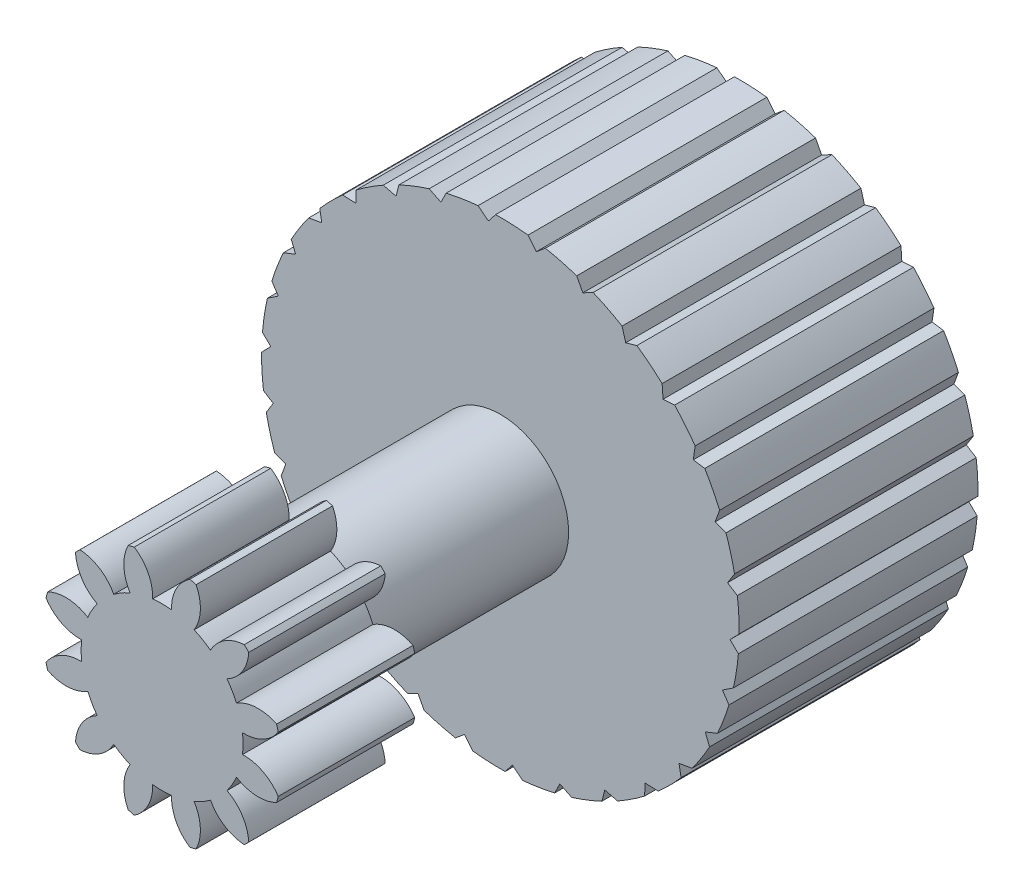
from build123d import *

# Parameters (mm, degrees)
SKETCH1_R           = 1
BOSS_EXTRUDE1_DEPTH = 3
BOSS_EXTRUDE2_DEPTH = 2
SKETCH3_R           = 3.5
BOSS_EXTRUDE3_DEPTH = 3.5
CUT_EXTRUDE1_DEPTH  = 5
CIRPATTERN1_COUNT   = 30
SCALE_1_SCALE       = 0.7


with BuildPart() as part:
    # Sketch1 → Boss-Extrude1 (new body)
    with BuildSketch(Plane.XY):
        Circle(SKETCH1_R)
    extrude(amount=BOSS_EXTRUDE1_DEPTH)

    # Sketch2 → Boss-Extrude2 (add)
    with BuildSketch(Plane.XY.offset(3)):
        with BuildLine():
            ThreePointArc((-1.227935913, 1.133778741), (-1.133506118, 0.844526988), (-0.90932576, 0.638792379))
            ThreePointArc((-0.90932576, 0.638792379), (-0.985601146, 0.522902394), (-1.047827124, 0.39890098))
            ThreePointArc((-1.047827124, 0.39890098), (-1.338088701, 0.490179561), (-1.635802964, 0.427332285))
            ThreePointArc((-1.635802964, 0.427332285), (-1.6484322, 0.382585723), (-1.659868241, 0.337519445))
            ThreePointArc((-1.659868241, 0.337519445), (-1.433463765, 0.134234977), (-1.136450575, 0.068153758))
            ThreePointArc((-1.136450575, 0.068153758), (-1.144562004, -0.070347606), (-1.136450575, -0.208848969))
            ThreePointArc((-1.136450575, -0.208848969), (-1.433463765, -0.274930188), (-1.659868241, -0.478214657))
            ThreePointArc((-1.659868241, -0.478214657), (-1.6484322, -0.523280934), (-1.635802964, -0.568027497))
            ThreePointArc((-1.635802964, -0.568027497), (-1.338088701, -0.630874772), (-1.047827124, -0.539596191))
            ThreePointArc((-1.047827124, -0.539596191), (-0.985601146, -0.663597606), (-0.90932576, -0.77948759))
            ThreePointArc((-0.90932576, -0.77948759), (-1.133506118, -0.985222199), (-1.227935913, -1.274473952))
            ThreePointArc((-1.227935913, -1.274473952), (-1.195498871, -1.307784473), (-1.16218835, -1.340221514))
            ThreePointArc((-1.16218835, -1.340221514), (-0.872936598, -1.24579172), (-0.667201989, -1.021611361))
            ThreePointArc((-0.667201989, -1.021611361), (-0.551312004, -1.097886747), (-0.42731059, -1.160112725))
            ThreePointArc((-0.42731059, -1.160112725), (-0.518589171, -1.450374302), (-0.455741895, -1.748088565))
            ThreePointArc((-0.455741895, -1.748088565), (-0.410995333, -1.760717802), (-0.365929055, -1.772153843))
            ThreePointArc((-0.365929055, -1.772153843), (-0.162644586, -1.545749366), (-0.096563368, -1.248736176))
            ThreePointArc((-0.096563368, -1.248736176), (0.041937996, -1.256847606), (0.180439359, -1.248736176))
            ThreePointArc((0.180439359, -1.248736176), (0.246520578, -1.545749366), (0.449805047, -1.772153843))
            ThreePointArc((0.449805047, -1.772153843), (0.494871325, -1.760717802), (0.539617887, -1.748088565))
            ThreePointArc((0.539617887, -1.748088565), (0.602465162, -1.450374302), (0.511186581, -1.160112725))
            ThreePointArc((0.511186581, -1.160112725), (0.635187996, -1.097886747), (0.75107798, -1.021611361))
            ThreePointArc((0.75107798, -1.021611361), (0.956812589, -1.24579172), (1.246064342, -1.340221514))
            ThreePointArc((1.246064342, -1.340221514), (1.279374863, -1.307784473), (1.311811904, -1.274473952))
            ThreePointArc((1.311811904, -1.274473952), (1.21738211, -0.985222199), (0.993201751, -0.77948759))
            ThreePointArc((0.993201751, -0.77948759), (1.069477137, -0.663597606), (1.131703115, -0.539596191))
            ThreePointArc((1.131703115, -0.539596191), (1.421964692, -0.630874772), (1.719678955, -0.568027497))
            ThreePointArc((1.719678955, -0.568027497), (1.732308192, -0.523280934), (1.743744233, -0.478214657))
            ThreePointArc((1.743744233, -0.478214657), (1.517339756, -0.274930188), (1.220326566, -0.208848969))
            ThreePointArc((1.220326566, -0.208848969), (1.228437996, -0.070347606), (1.220326566, 0.068153758))
            ThreePointArc((1.220326566, 0.068153758), (1.517339756, 0.134234977), (1.743744233, 0.337519445))
            ThreePointArc((1.743744233, 0.337519445), (1.732308192, 0.382585723), (1.719678955, 0.427332285))
            ThreePointArc((1.719678955, 0.427332285), (1.421964692, 0.490179561), (1.131703115, 0.39890098))
            ThreePointArc((1.131703115, 0.39890098), (1.069477137, 0.522902394), (0.993201751, 0.638792379))
            ThreePointArc((0.993201751, 0.638792379), (1.21738211, 0.844526988), (1.311811904, 1.133778741))
            ThreePointArc((1.311811904, 1.133778741), (1.279374863, 1.167089262), (1.246064342, 1.199526303))
            ThreePointArc((1.246064342, 1.199526303), (0.956812589, 1.105096508), (0.75107798, 0.88091615))
            ThreePointArc((0.75107798, 0.88091615), (0.635187996, 0.957191536), (0.511186581, 1.019417514))
            ThreePointArc((0.511186581, 1.019417514), (0.602465162, 1.309679091), (0.539617887, 1.607393354))
            ThreePointArc((0.539617887, 1.607393354), (0.494871325, 1.62002259), (0.449805047, 1.631458632))
            ThreePointArc((0.449805047, 1.631458632), (0.246520578, 1.405054155), (0.180439359, 1.108040965))
            ThreePointArc((0.180439359, 1.108040965), (0.041937996, 1.116152394), (-0.096563368, 1.108040965))
            ThreePointArc((-0.096563368, 1.108040965), (-0.162644586, 1.405054155), (-0.365929055, 1.631458632))
            ThreePointArc((-0.365929055, 1.631458632), (-0.410995333, 1.62002259), (-0.455741895, 1.607393354))
            ThreePointArc((-0.455741895, 1.607393354), (-0.518589171, 1.309679091), (-0.42731059, 1.019417514))
            ThreePointArc((-0.42731059, 1.019417514), (-0.551312004, 0.957191536), (-0.667201989, 0.88091615))
            ThreePointArc((-0.667201989, 0.88091615), (-0.872936598, 1.105096508), (-1.16218835, 1.199526303))
            ThreePointArc((-1.16218835, 1.199526303), (-1.195498871, 1.167089262), (-1.227935913, 1.133778741))
        make_face()
    extrude(amount=BOSS_EXTRUDE2_DEPTH)

    # Sketch3 → Boss-Extrude3 (add)
    with BuildSketch(Plane(origin=(0, 0, 0), x_dir=(-1, 0, 0), z_dir=(0, 0, -1))):
        Circle(SKETCH3_R)
    extrude(amount=BOSS_EXTRUDE3_DEPTH)

    # Sketch4 → Cut-Extrude1 (cut)
    with BuildSketch(Plane(origin=(0, 0, -3.5), x_dir=(-1, 0, 0), z_dir=(0, 0, -1))):
        Polygon((0.070137448, 3.499297178), (0.175445666, 3.365353505), (0.327208501, 3.484671376), (0.327208501, 3.816079959), (0.070137448, 3.816079959), align=None)
    cut_extrude1 = extrude(amount=-CUT_EXTRUDE1_DEPTH, mode=Mode.SUBTRACT)

    # CirPattern1: Cut-Extrude1 ×30 about axis
    cirpattern1_axis = Axis((0, 0, 0), (0, 0, 1))
    for i in range(1, CIRPATTERN1_COUNT):
        add(cut_extrude1.rotate(cirpattern1_axis, i * 360 / CIRPATTERN1_COUNT), mode=Mode.SUBTRACT)


with BuildPart() as part_1:
    # Scale 1: scaled about (0, 0, 0)
    add(part.part.scale(SCALE_1_SCALE))


solid = part_1.part
